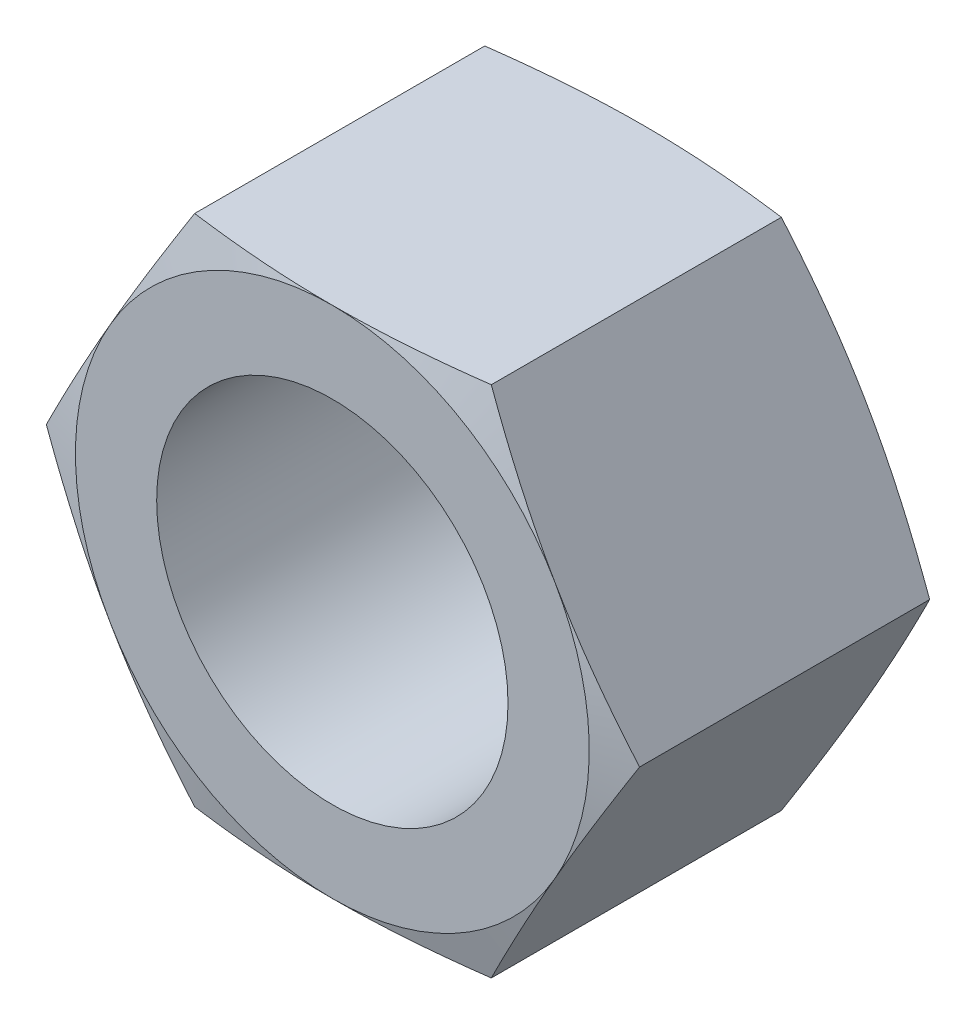
from build123d import *

# Parameters (mm, degrees)
SKETCH1_R          = 18
BASE_EXTRUDE_DEPTH = 31.9
SKETCH2_OUTSIDE_W  = 363.728
SKETCH2_OUTSIDE_H  = 355.584
SKETCH2_OUTSIDE_R  = 26.322842148
CUT_EXTRUDE1_DEPTH = 38
CUT_EXTRUDE1_DRAFT = -75
SKETCH3_OUTSIDE_W  = 363.728
SKETCH3_OUTSIDE_H  = 355.584
SKETCH3_OUTSIDE_R  = 26.322842148
CUT_EXTRUDE2_DEPTH = 38
CUT_EXTRUDE2_DRAFT = -75


with BuildPart() as part:
    # Sketch1 → Base-Extrude (new body)
    with BuildSketch(Plane.XY):
        Polygon((15.1975, 26.322842148), (-15.1975, 26.322842148), (-30.395, 0), (-15.1975, -26.322842148), (15.1975, -26.322842148), (30.395, 0), align=None)
        Circle(SKETCH1_R, mode=Mode.SUBTRACT)
    extrude(amount=BASE_EXTRUDE_DEPTH)


with BuildPart() as cut_extrude1_tool:
    # Sketch2 outside → Cut-Extrude1 (with draft: the straight prism first)
    with BuildSketch(Plane(origin=(0, 0, 0), x_dir=(-1, 0, 0), z_dir=(0, 0, -1))):
        Rectangle(SKETCH2_OUTSIDE_W, SKETCH2_OUTSIDE_H)
        Circle(SKETCH2_OUTSIDE_R, mode=Mode.SUBTRACT)
    extrude(amount=-CUT_EXTRUDE1_DEPTH)
    # Cut-Extrude1: the draft: its side faces are tilted about the plane it starts from
    cut_extrude1_sides = [cut_extrude1_tool.faces().sort_by_distance(p)[0] for p in [
        (0, -177.792, 19),
        (-181.864, 0, 19),
        (0, 177.792, 19),
        (181.864, 0, 19),
        (26.322842148, 0, 19),
    ]]
    draft(cut_extrude1_sides, Plane(origin=(0, 0, 0), x_dir=(-1, 0, 0), z_dir=(0, 0, -1)), CUT_EXTRUDE1_DRAFT)


with BuildPart() as part_1:
    add(part.part)

    # Cut-Extrude1: cut by cut_extrude1_tool
    add(cut_extrude1_tool.part, mode=Mode.SUBTRACT)


with BuildPart() as cut_extrude2_tool:
    # Sketch3 outside → Cut-Extrude2 (with draft: the straight prism first)
    with BuildSketch(Plane.XY.offset(31.9)):
        Rectangle(SKETCH3_OUTSIDE_W, SKETCH3_OUTSIDE_H)
        Circle(SKETCH3_OUTSIDE_R, mode=Mode.SUBTRACT)
    extrude(amount=-CUT_EXTRUDE2_DEPTH)
    # Cut-Extrude2: the draft: its side faces are tilted about the plane it starts from
    cut_extrude2_sides = [cut_extrude2_tool.faces().sort_by_distance(p)[0] for p in [
        (0, -177.792, 12.9),
        (181.864, 0, 12.9),
        (0, 177.792, 12.9),
        (-181.864, 0, 12.9),
        (-26.322842148, 0, 12.9),
    ]]
    draft(cut_extrude2_sides, Plane.XY.offset(31.9), CUT_EXTRUDE2_DRAFT)


with BuildPart() as part_2:
    add(part_1.part)

    # Cut-Extrude2: cut by cut_extrude2_tool
    add(cut_extrude2_tool.part, mode=Mode.SUBTRACT)


solid = part_2.part
